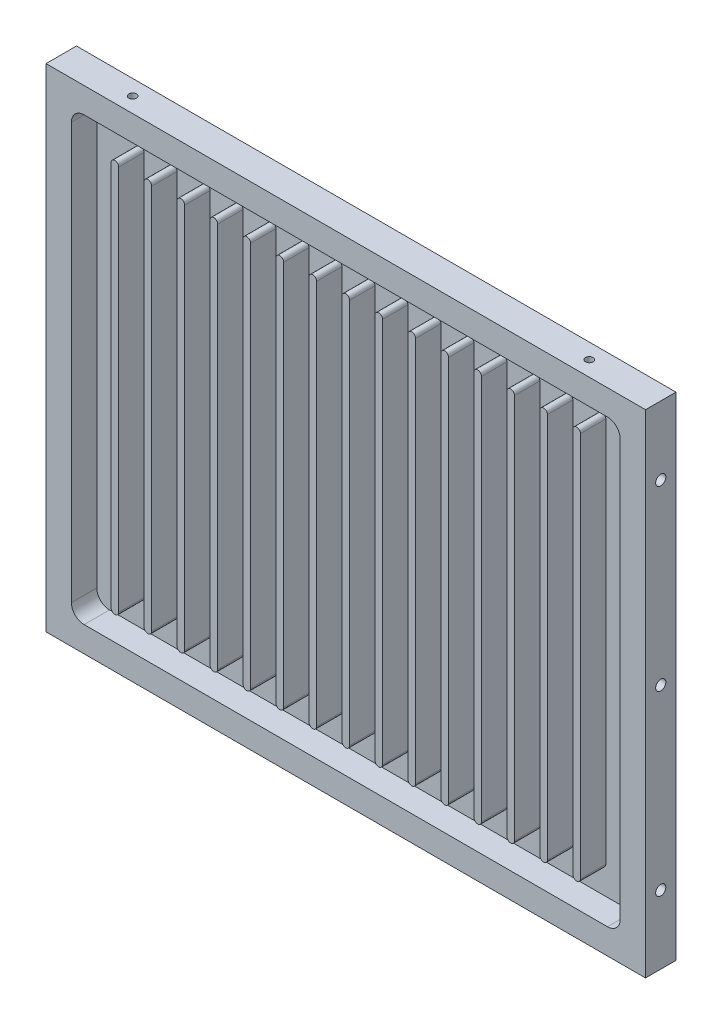
SolidWorks part; units mm, degrees
ref_plane "Front Plane" through (0, 0, 0) normal (0, 0, 1) x (1, 0, 0)
ref_plane "Top Plane" through (0, 0, 0) normal (0, 1, 0) x (1, 0, 0)
ref_plane "Right Plane" through (0, 0, 0) normal (1, 0, 0) x (0, 0, -1)
sketch "Sketch1" plane through (0, 0, 0) normal (0, 0, 1) x (1, 0, 0)
  line L1 (-118.15, 97) -> (118.15, 97)
  line L2 (-118.15, 97) -> (-118.15, -97)
  line L3 (-118.15, -97) -> (118.15, -97)
  line L4 (118.15, 97) -> (118.15, -97)
  line L5 (-118.15, 97) -> (118.15, -97) construction
  line L6 (-118.15, -97) -> (118.15, 97) construction
  point P0 (0, 0)
  dimension "D1" = 236.3
  dimension "D2" = 194
extrude "Boss-Extrude1" add sketch "Sketch1" along normal mid plane 12
sketch "Sketch2" plane through (0, 0, 6) normal (0, 0, 1) x (1, 0, 0)
  line L8 (108.15, -87) -> (108.15, 87)
  line L9 (108.15, 87) -> (-108.15, 87)
  line L10 (-108.15, 87) -> (-108.15, -87)
  line L11 (-108.15, -87) -> (108.15, -87)
  line L12 (108.15, -87) -> (108.15, 87)
  line L13 (108.15, 87) -> (-108.15, 87)
  line L14 (-108.15, 87) -> (-108.15, -87)
  line L15 (-108.15, -87) -> (108.15, -87)
  dimension "D1" = 10
extrude "Cut-Extrude1" cut sketch "Sketch2" against normal blind 10 from surface at 0 starting at face at (0, 0, 6)
sketch "Sketch3" plane through (0, 0, -4) normal (0, 0, 1) x (1, 0, 0)
  line L0 (-2.366, 0) -> (2.2741, 0) construction
  line L1 (-0.5, 77.5) -> (0.5, 77.5) construction
  line L2 (-1.5, 76) -> (-1.5, -76)
  line L3 (-0.5, -77.5) -> (0.5, -77.5) construction
  line L4 (1.5, 76) -> (1.5, -76)
  line L5 (-1.5, 77.5) -> (1.5, -77.5) construction
  line L6 (-1.5, -77.5) -> (1.5, 77.5) construction
  arc A0 (0.5, -77.5) -> (1.5, -76.5) centre (0.5, -76.5) ccw construction
  arc A1 (-1.5, -76.5) -> (-0.5, -77.5) centre (-0.5, -76.5) ccw construction
  arc A2 (0.5, 77.5) -> (1.5, 76.5) centre (0.5, 76.5) cw construction
  arc A3 (-0.5, 77.5) -> (-1.5, 76.5) centre (-0.5, 76.5) ccw construction
  arc A4 (1.5, 76) -> (-1.5, 76) centre (0, 76) ccw
  arc A5 (1.5, -76) -> (-1.5, -76) centre (0, -76) cw
  point P0 (0, 0)
  dimension "D3" = 1
  dimension "D4" = 3
  dimension "D1" = 3
  dimension "D2" = 155
extrude "Boss-Extrude2" add sketch "Sketch3" along normal blind 10
pattern_linear "LPattern1" count 8 spacing 13 along (1, 0, 0) count 8 spacing 13 along (-1, 0, 0) seed only of "Boss-Extrude2"
sketch "Sketch5" plane through (0, 97, 0) normal (0, 1, 0) x (1, 0, 0)
  line L0 (-143.645, 0) -> (131.7839, 0) construction
  line L1 (0, 20.7848) -> (0, -27.2459) construction
  line L2 (118.15, -6) -> (-118.15, -6) construction
  circle A0 centre (-90, 0) radius 1.5
  circle A1 centre (90, 0) radius 1.5
  dimension "D1" = 3
  dimension "D2" = 90
  dimension "D3" = 6
extrude "Cut-Extrude2" cut sketch "Sketch5" against normal blind 4
mirror "Mirror1" about plane through (0, 0, 0) normal (0, 1, 0) of "Cut-Extrude2"
sketch "Sketch6" plane through (-118.15, 0, 0) normal (-1, 0, 0) x (0, 0, 1)
  line L0 (-31.2906, 0) -> (48.6902, 0) construction
  line L1 (6, 97) -> (6, -97) construction
  circle A0 centre (0, 70) radius 2
  circle A1 centre (0, 0) radius 2
  circle A2 centre (0, -70) radius 2
  dimension "D1" = 4
  dimension "D2" = 6
  dimension "D3" = 70
  dimension "D4" = 4
  dimension "D5" = 6
extrude "Cut-Extrude3" cut sketch "Sketch6" against normal blind 4
mirror "Mirror2" about plane through (0, 0, 0) normal (1, 0, 0) of "Cut-Extrude3"
fillet "Fillet1" radius 5 4 edges at (108.15, 87, 1) (108.15, -87, 1) (-108.15, -87, 1) (-108.15, 87, 1)
